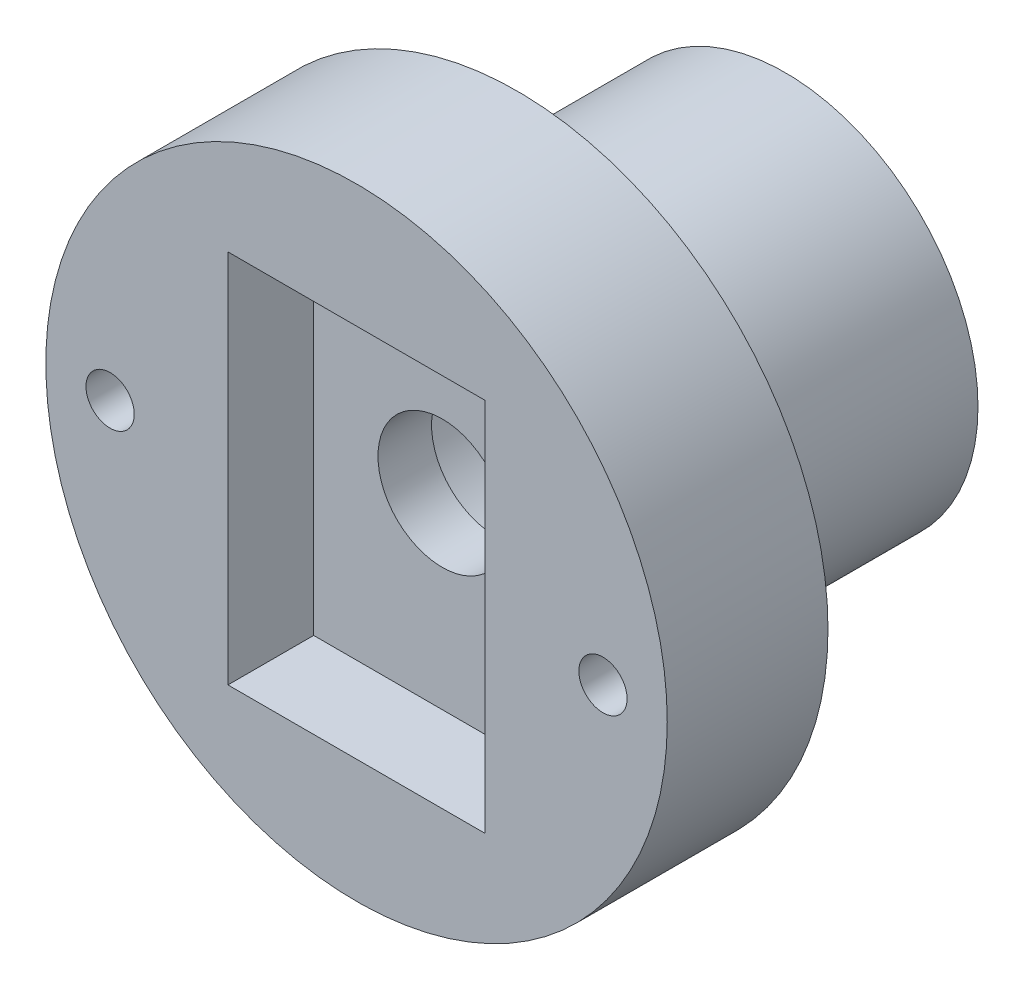
SolidWorks part; units mm, degrees
ref_plane "前视基准面" through (0, 0, 0) normal (0, 0, 1) x (1, 0, 0)
ref_plane "上视基准面" through (0, 0, 0) normal (0, 1, 0) x (1, 0, 0)
ref_plane "右视基准面" through (0, 0, 0) normal (1, 0, 0) x (0, 0, -1)
sketch "草图1" plane through (0, 0, 0) normal (0, 0, 1) x (1, 0, 0)
  circle A0 centre (0, 0) radius 11
  circle A1 centre (0, 0) radius 18
  dimension "D1" = 22
  dimension "D2" = 36
extrude "凸台-拉伸1" add sketch "草图1" along normal blind 25
sketch "草图2" plane through (0, 0, 25) normal (0, 0, 1) x (1, 0, 0)
  circle A0 centre (0, 0) radius 11
  circle A1 centre (0, 0) radius 29
  circle A2 centre (0, 0) radius 11 construction
  circle A3 centre (0, 0) radius 18 construction
  dimension "D1" = 58
extrude "凸台-拉伸2" add sketch "草图2" along normal blind 15
hole_wizard "打孔尺寸根据内六角圆柱头螺钉的类型1" positions "草图4" profile "草图3" counterbore size "M4" standard "Gb" end condition through all
sketch "草图4" plane through (0, 0, 25) normal (0, 0, -1) x (-1, 0, 0)
  point P0 (-23, 0)
  point P2 (23, 0)
  dimension "D1" = 23
  dimension "D2" = 23
sketch "草图3" plane through (23, 0, 25) normal (1, 0, 0) x (0, 1, 0)
  line L0 (0, 0) -> (0, 15)
  line L1 (0, 15) -> (2.25, 15)
  line L3 (2.25, 15) -> (2.25, 4.6)
  line L4 (2.25, 4.6) -> (4, 4.6)
  line L5 (4, 4.6) -> (4, 0)
  line L7 (4, 0) -> (0, 0)
  line L11 (0, -6.35) -> (0, 107.95) construction
  dimension "通孔孔直径" = 4.5
  dimension "通孔孔深度" = 15
  dimension "柱形沉头孔直径" = 8
  dimension "柱形沉头孔深度" = 4.6
sketch "草图6" plane through (0, 0, 40) normal (0, 0, 1) x (1, 0, 0)
  line L1 (-12, 17.5) -> (12, 17.5)
  line L2 (-12, 17.5) -> (-12, -17.5)
  line L3 (-12, -17.5) -> (12, -17.5)
  line L4 (12, 17.5) -> (12, -17.5)
  line L5 (-12, 17.5) -> (12, -17.5) construction
  line L6 (-12, -17.5) -> (12, 17.5) construction
  point P0 (0, 0)
  dimension "D1" = 24
  dimension "D2" = 35
extrude "切除-拉伸1" cut sketch "草图6" against normal blind 8
sketch "草图7" plane through (0, 0, 32) normal (0, 0, 1) x (1, 0, 0)
  circle A0 centre (0, 0) radius 11
  circle A1 centre (0, 0) radius 6
  dimension "D1" = 12
  dimension "D2" = 22
extrude "凸台-拉伸3" add sketch "草图7" against normal blind 5
